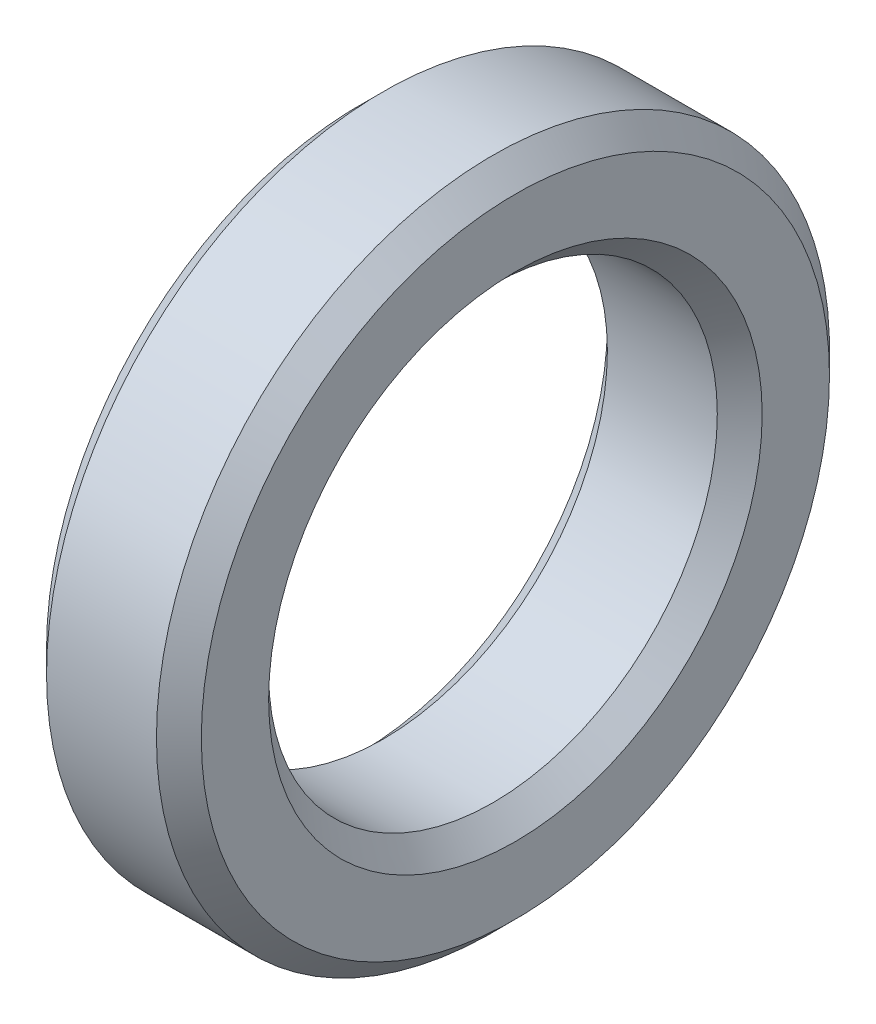
from build123d import *

# Parameters (mm, degrees)
SKETCH1_R           = 15
SKETCH1_R_2         = 10
BOSS_EXTRUDE1_DEPTH = 6.9
CHAMFER1_SIZE       = 1


with BuildPart() as part:
    # Sketch1 → Boss-Extrude1 (new body)
    with BuildSketch(Plane(origin=(0, 0, 0), x_dir=(0, 0, -1), z_dir=(1, 0, 0))):
        with Locations(Location((0, 0, 0), (0, 0, 180))):
            Circle(SKETCH1_R)
        with Locations(Location((0, 0, 0), (0, 0, 180))):
            Circle(SKETCH1_R_2, mode=Mode.SUBTRACT)
    extrude(amount=BOSS_EXTRUDE1_DEPTH)

    # Chamfer1
    chamfer1_edges = [part.edges().sort_by_distance(p)[0] for p in [
        (0, 0, -15),
        (6.9, 0, -15),
        (0, 0, -10),
        (6.9, 0, -10),
    ]]
    chamfer(chamfer1_edges, length=CHAMFER1_SIZE)


solid = part.part
